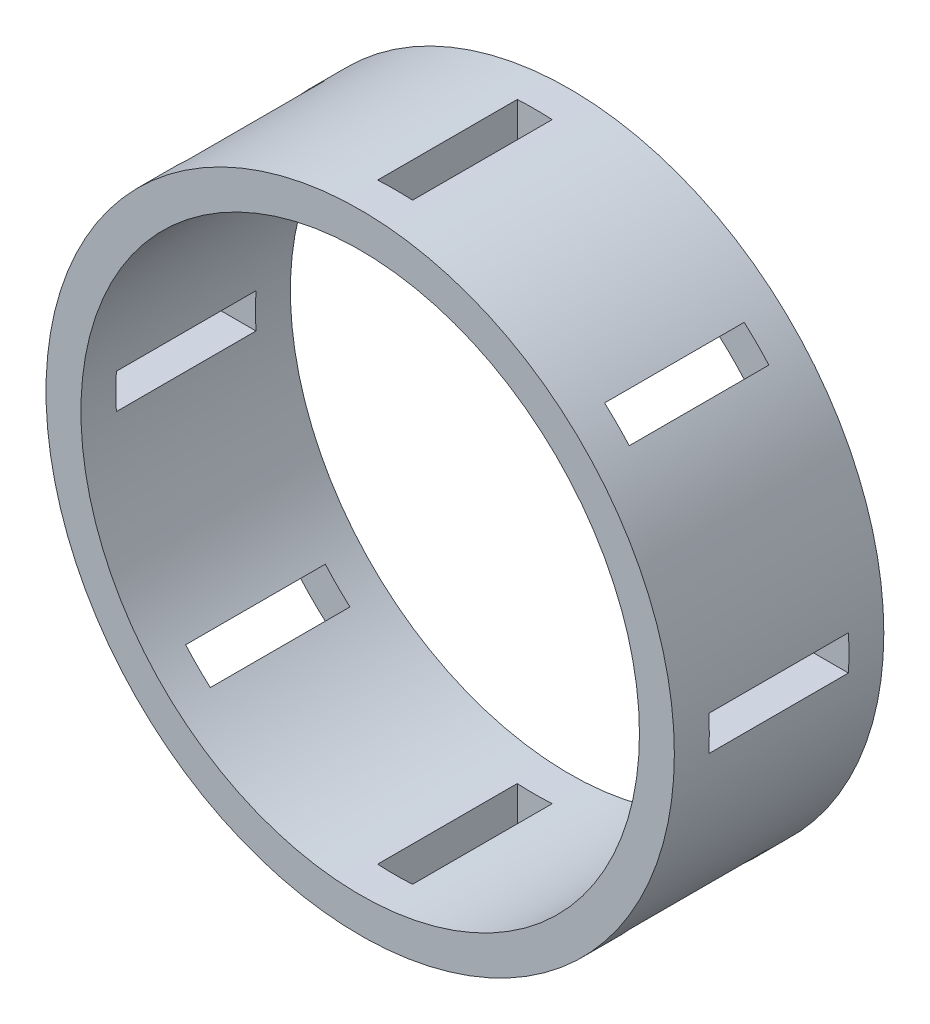
SolidWorks part; units mm, degrees
ref_plane "Front Plane" through (0, 0, 0) normal (0, 0, 1) x (1, 0, 0)
ref_plane "Top Plane" through (0, 0, 0) normal (0, 1, 0) x (1, 0, 0)
ref_plane "Right Plane" through (0, 0, 0) normal (1, 0, 0) x (0, 0, -1)
other "Configuration Table"
sketch "Sketch1" plane through (0, 0, 0) normal (0, 0, 1) x (1, 0, 0)
  circle A0 centre (-599.8842, -90) radius 45
  circle A1 centre (-599.8842, -90) radius 40
  dimension "D1" = 90
  dimension "D2" = 80
extrude "Boss-Extrude1" add sketch "Sketch1" along normal blind 30
sketch "Sketch2" plane through (0, 0, 0) normal (0, 1, 0) x (1, 0, 0)
  line L0 (-599.8842, -30) -> (-599.8842, 0) construction
  line L1 (-602.3842, -25) -> (-597.3842, -25)
  line L2 (-602.3842, -25) -> (-602.3842, -5)
  line L3 (-602.3842, -5) -> (-597.3842, -5)
  line L4 (-597.3842, -25) -> (-597.3842, -5)
  line L5 (-602.3842, -25) -> (-597.3842, -5) construction
  line L6 (-602.3842, -5) -> (-597.3842, -25) construction
  line L7 (-644.8842, -15) -> (-586.5805, -15) construction
  line L8 (-644.8842, 0) -> (-644.8842, -30) construction
  point P0 (-599.8842, -15)
  dimension "D1" = 20
  dimension "D2" = 5
extrude "Cut-Extrude1" cut sketch "Sketch2" against normal through all both and the other way through all
pattern_circular "CirPattern1" count 8 over 360 about axis through (-599.8842, -90, 0) along (0, 0, 1) of "Cut-Extrude1"
